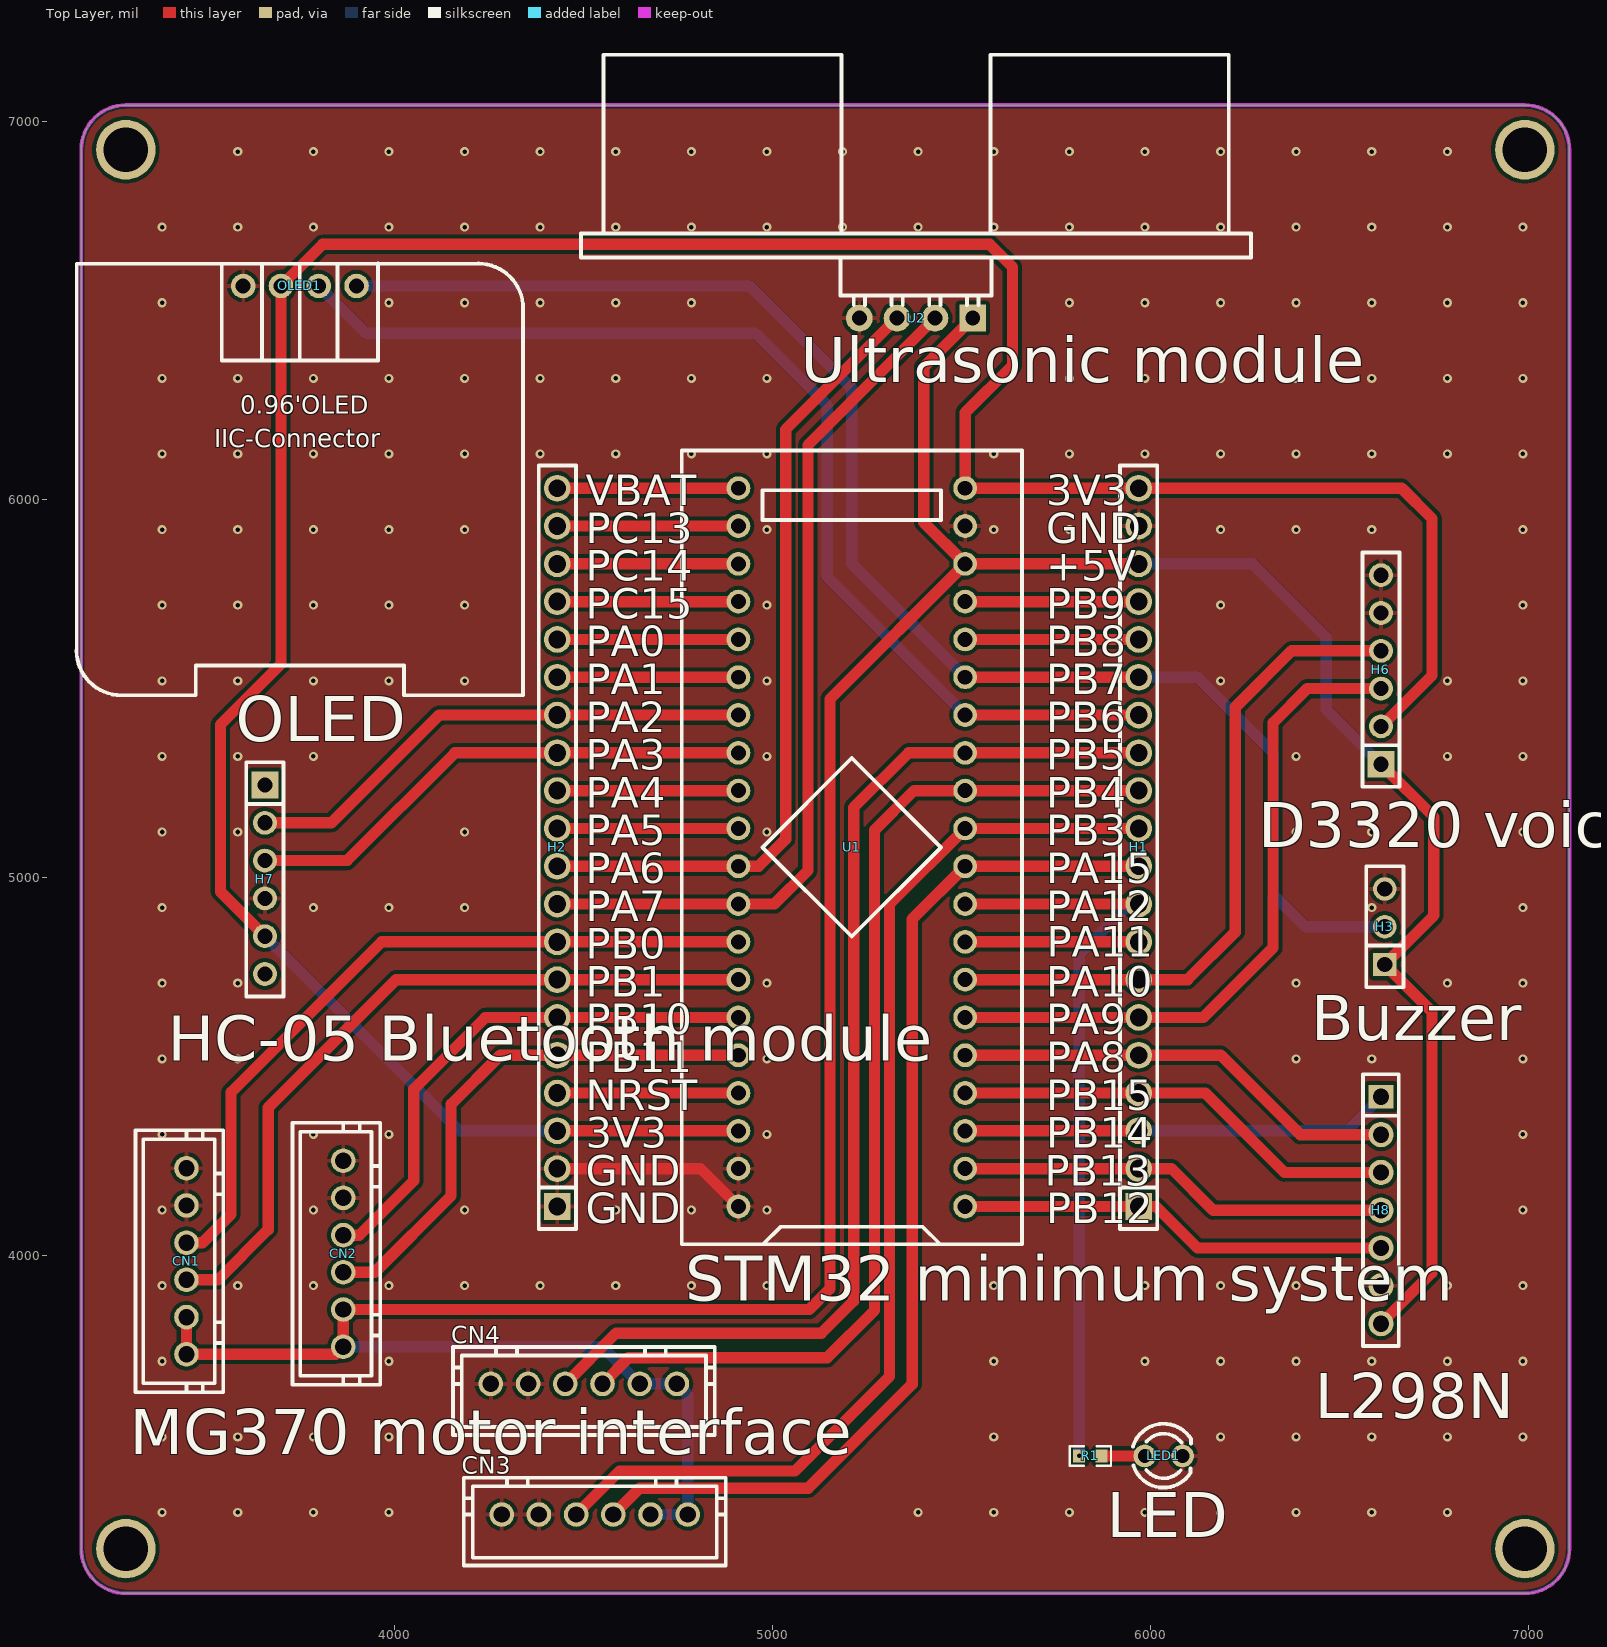
[diagram p0: Top Layer view]
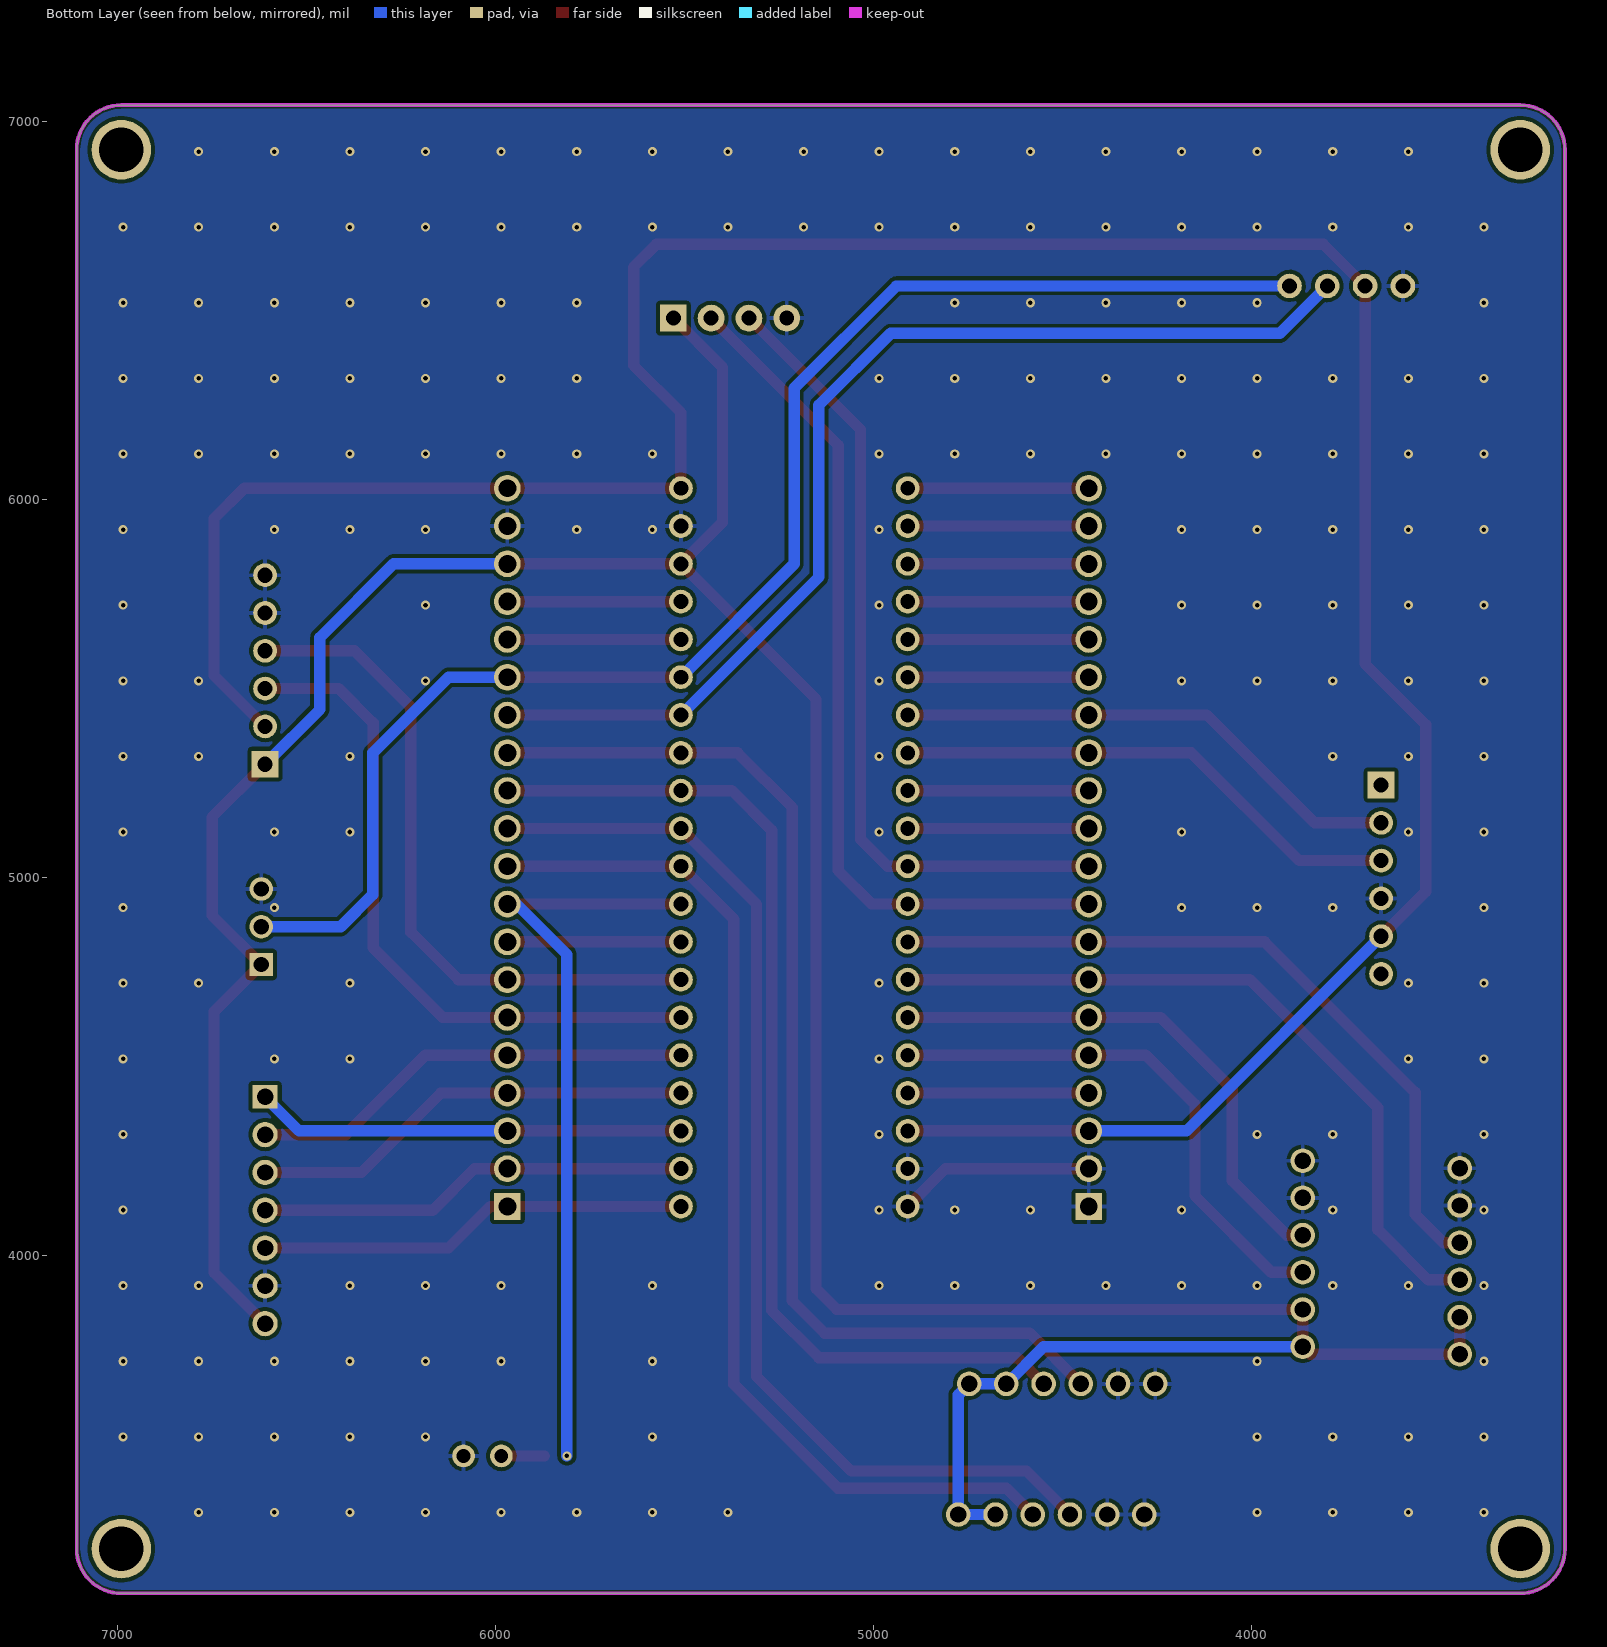
[diagram p1: Bottom Layer view, seen from below]
# Altium PCB MISC89099.pcbdoc
Units mil, origin at the board's own origin, x right, y up, seen from the top; angles counter-clockwise.
Board outline 3937.01 x 3937.01 mil, 2 copper layers (Top Layer, Bottom Layer), stack 62.206 mil thick; 15 components, 38 nets, 142 pads, 202 vias.

## Layer stack, top to bottom
Top Solder Mask Layer: solder mask 0.394, Dk 3.3
Top Layer: signal copper 1.379
Dielectric1: surface 59.449, FR4, Dk 4.5
Bottom Layer: signal copper 1.378
Bottom Solder Mask Layer: solder mask 0.394, Dk 3.3

## Board outline
3289.61,7043.5 ccw(c3289.61,6925.39) 3171.5,6925.39 3171.5,3224.61 ccw(c3289.61,3224.61) 3289.61,3106.5 6990.39,3106.5 ccw(c6990.39,3224.61) 7108.5,3224.61 7108.5,6925.39 ccw(c6990.39,6925.39) 6990.39,7043.5 3289.61,7043.5

## Design rules (kind name [scope] priority, off if disabled: settings)
BoardOutlineClearance copperThickness2oz_1 [All] p2 off: genericclearance=7.99 ignorepadtopadclearanceinfootprint=FALSE except(0: Arc-SplitContinuation Track-SplitContinuation SMDPad-SplitContinuation THPad-SplitContinuation Via-SplitContinuation Fill-SplitContinuation Region-SplitContinuation Poly-SplitContinuation Text-SplitContinuation Hole-SplitContinuation; 5.98: Arc-CutoutEdge Track-CutoutEdge SMDPad-CutoutEdge THPad-CutoutEdge Via-CutoutEdge Text-CutoutEdge; 6.9: Hole-OutlineEdge Hole-CutoutEdge; 10: Poly-OutlineEdge Poly-CutoutEdge; 11.81: Arc-OutlineEdge Track-OutlineEdge SMDPad-OutlineEdge THPad-OutlineEdge Via-OutlineEdge Fill-OutlineEdge Region-OutlineEdge Text-OutlineEdge Fill-CutoutEdge Region-CutoutEdge)
BoardOutlineClearance Plane_innerPlane_1 [All] p4 off: genericclearance=4.02 ignorepadtopadclearanceinfootprint=FALSE except(0: Arc-SplitContinuation Track-SplitContinuation SMDPad-SplitContinuation THPad-SplitContinuation Via-SplitContinuation Fill-SplitContinuation Region-SplitContinuation Poly-SplitContinuation Text-SplitContinuation Hole-SplitContinuation; 5.98: Arc-CutoutEdge Track-CutoutEdge SMDPad-CutoutEdge THPad-CutoutEdge Via-CutoutEdge Text-CutoutEdge; 6.9: Hole-OutlineEdge Hole-CutoutEdge; 10: Poly-OutlineEdge Poly-CutoutEdge; 11.81: Arc-OutlineEdge Track-OutlineEdge SMDPad-OutlineEdge THPad-OutlineEdge Via-OutlineEdge Fill-OutlineEdge Region-OutlineEdge Text-OutlineEdge Fill-CutoutEdge Region-CutoutEdge)
BoardOutlineClearance Copper_copperRegion_1 [All] p6 off: genericclearance=4.02 ignorepadtopadclearanceinfootprint=FALSE except(0: Arc-SplitContinuation Track-SplitContinuation SMDPad-SplitContinuation THPad-SplitContinuation Via-SplitContinuation Fill-SplitContinuation Region-SplitContinuation Poly-SplitContinuation Text-SplitContinuation Hole-SplitContinuation; 5.98: Arc-CutoutEdge Track-CutoutEdge SMDPad-CutoutEdge THPad-CutoutEdge Via-CutoutEdge Text-CutoutEdge; 6.9: Hole-OutlineEdge Hole-CutoutEdge; 10: Poly-OutlineEdge Poly-CutoutEdge; 11.81: Arc-OutlineEdge Track-OutlineEdge SMDPad-OutlineEdge THPad-OutlineEdge Via-OutlineEdge Fill-OutlineEdge Region-OutlineEdge Text-OutlineEdge Fill-CutoutEdge Region-CutoutEdge)
BoardOutlineClearance copperThickness1oz_1 [All] p8: genericclearance=4.02 ignorepadtopadclearanceinfootprint=FALSE except(0: Arc-SplitContinuation Track-SplitContinuation SMDPad-SplitContinuation THPad-SplitContinuation Via-SplitContinuation Fill-SplitContinuation Region-SplitContinuation Poly-SplitContinuation Text-SplitContinuation Hole-SplitContinuation; 5.98: Arc-CutoutEdge Track-CutoutEdge SMDPad-CutoutEdge THPad-CutoutEdge Via-CutoutEdge Text-CutoutEdge; 6.9: Hole-OutlineEdge Hole-CutoutEdge; 10: Poly-OutlineEdge Poly-CutoutEdge; 11.81: Arc-OutlineEdge Track-OutlineEdge SMDPad-OutlineEdge THPad-OutlineEdge Via-OutlineEdge Fill-OutlineEdge Region-OutlineEdge Text-OutlineEdge Fill-CutoutEdge Region-CutoutEdge)
Clearance copperThickness2oz [All] p1 off: gap=7.99 ignorepadtopadclearanceinfootprint=FALSE except(5.98: SMDPad-Track SMDPad-SMDPad THPad-Track SMDPad-THPad THPad-THPad Track-Via SMDPad-Via THPad-Via Via-Via Fill-SMDPad Region-SMDPad Fill-THPad Region-THPad Fill-Via Region-Via Fill-Fill Fill-Region Region-Region Arc-Track Arc-SMDPad Arc-THPad Arc-Via Fill-Arc Region-Arc Arc-Arc Text-Track SMDPad-Text Text-THPad Text-Via Fill-Text Region-Text Arc-Text Text-Text; 6.9: Hole-Track Hole-SMDPad Hole-THPad Hole-Via Fill-Hole Region-Hole Hole-Arc Hole-Text; 10: Poly-Track Poly-SMDPad Poly-THPad Poly-Via Poly-Fill Poly-Region Poly-Poly Poly-Arc Poly-Text Poly-Hole; 11.81: Fill-Track Region-Track)
Clearance Plane_innerPlane [All] p3 off: gap=4.02 ignorepadtopadclearanceinfootprint=FALSE except(5.98: SMDPad-Track SMDPad-SMDPad THPad-Track SMDPad-THPad THPad-THPad Track-Via SMDPad-Via THPad-Via Via-Via Fill-SMDPad Region-SMDPad Fill-THPad Region-THPad Fill-Via Region-Via Fill-Fill Fill-Region Region-Region Arc-Track Arc-SMDPad Arc-THPad Arc-Via Fill-Arc Region-Arc Arc-Arc Text-Track SMDPad-Text Text-THPad Text-Via Fill-Text Region-Text Arc-Text Text-Text; 6.9: Hole-Track Hole-SMDPad Hole-THPad Hole-Via Fill-Hole Region-Hole Hole-Arc Hole-Text; 10: Poly-Track Poly-SMDPad Poly-THPad Poly-Via Poly-Fill Poly-Region Poly-Poly Poly-Arc Poly-Text Poly-Hole; 11.81: Fill-Track Region-Track)
Clearance Copper_copperRegion [All] p5 off: gap=4.02 ignorepadtopadclearanceinfootprint=FALSE except(5.98: SMDPad-Track SMDPad-SMDPad THPad-Track SMDPad-THPad THPad-THPad Track-Via SMDPad-Via THPad-Via Via-Via Fill-SMDPad Region-SMDPad Fill-THPad Region-THPad Fill-Via Region-Via Fill-Fill Fill-Region Region-Region Arc-Track Arc-SMDPad Arc-THPad Arc-Via Fill-Arc Region-Arc Arc-Arc Text-Track SMDPad-Text Text-THPad Text-Via Fill-Text Region-Text Arc-Text Text-Text; 6.9: Hole-Track Hole-SMDPad Hole-THPad Hole-Via Fill-Hole Region-Hole Hole-Arc Hole-Text; 10: Poly-Track Poly-SMDPad Poly-THPad Poly-Via Poly-Fill Poly-Region Poly-Poly Poly-Arc Poly-Text Poly-Hole; 11.81: Fill-Track Region-Track)
Clearance copperThickness1oz [All] p7: gap=4.02 ignorepadtopadclearanceinfootprint=FALSE except(5.98: SMDPad-Track SMDPad-SMDPad THPad-Track SMDPad-THPad THPad-THPad Track-Via SMDPad-Via THPad-Via Via-Via Fill-SMDPad Region-SMDPad Fill-THPad Region-THPad Fill-Via Region-Via Fill-Fill Fill-Region Region-Region Arc-Track Arc-SMDPad Arc-THPad Arc-Via Fill-Arc Region-Arc Arc-Arc Text-Track SMDPad-Text Text-THPad Text-Via Fill-Text Region-Text Arc-Text Text-Text; 6.9: Hole-Track Hole-SMDPad Hole-THPad Hole-Via Fill-Hole Region-Hole Hole-Arc Hole-Text; 10: Poly-Track Poly-SMDPad Poly-THPad Poly-Via Poly-Fill Poly-Region Poly-Poly Poly-Arc Poly-Text Poly-Hole; 11.81: Fill-Track Region-Track)
DiffPairsRouting differentialPair [All] p1: maxlimit=6 minlimit=6 mostfreqgap=6 toplayer_minwidth=5 toplayer_prefwidth=10 toplayer_maxwidth=100 toplayer_mingap=6 toplayer_prefgap=6 toplayer_maxgap=6 bottomlayer_minwidth=5 bottomlayer_prefwidth=10 bottomlayer_maxwidth=100 bottomlayer_mingap=6 bottomlayer_prefgap=6 bottomlayer_maxgap=6 maxuncoupledlength=10
HoleToHoleClearance otherClearance [All] p1: gap=11.81 allowstackedmicrovias=TRUE
Length netLength [All] p1: minlimit=0 maxlimit=0
PasteMaskExpansion pasteMaskExpansion [All] p1: expansion=0
PlaneConnect innerPlane [All] p1: planeconnectstyle=Relief reliefexpansion=20 reliefentries=4 reliefconductorwidth=10 reliefairgap=10
PolygonConnect copperRegion [All] p1: connectstyle=Relief reliefconductorwidth=10 reliefentries=4 polygonreliefangle="90 Angle" airgapwidth=10 via.connectstyle=Relief via.reliefconductorwidth=10 via.reliefentries=4 via.polygonreliefangle="90 Angle" via.airgapwidth=10
RoutingVias viaSize [All] p1: holewidth=12.01 width=24.02 viastyle="Through Hole" minholewidth=11.81 minwidth=19.68 maxholewidth=248.03 maxwidth=393.7
SolderMaskExpansion solderMaskExpansion [IsVia] p1: expansion=-1000 istentingtop=TRUE
SolderMaskExpansion solderMaskExpansion [All] p2: expansion=2 istentingtop=FALSE
Width copperThickness2oz_2 [All] p1 off: maxlimit=100 minlimit=8 preferedwidth=10
Width copperThickness1oz_2 [All] p2: maxlimit=100 minlimit=5 preferedwidth=10

## Components (designator, comment, footprint, x,y, rotation, side; value= is the part's Value field where it differs from the comment)
CN1 "XH2.54*6P_through-hole" CONN-TH_XH2.54-6P 3450,3985 r270 top
CN2 "XH2.54*6P_through-hole" CONN-TH_XH2.54-6P 3865,4005 r270 top
CN3 "XH2.54*6P_through-hole" CONN-TH_XH2.54-6P 4530,3315 r0 top
CN4 "XH2.54*6P_through-hole" CONN-TH_XH2.54-6P 4501.36,3660.61 r0 top
H1 "" HDR-TH_20P-P2.54-V-F 5969.16,5080 r90 top
H2 "" HDR-TH_20P-P2.54-V-F 4430.95,5080 r90 top
H3 "" HDR-TH_3P-P2.54-V-F 6620,4870 r90 top
H6 "" HDR-TH_6P-P2.54-V-F 6610,5550 r90 top
H7 "" HDR-TH_6P-P2.54-V-F 3657.66,4995 r270 top
H8 "" HDR-TH_7P-P2.54-V-F 6610.01,4120 r270 top
LED1 "" LED_TH-3mm 6035,3470 r0 top
OLED1 "" 0.96OLED_4P 3750,6565 r0 top
R1 "220" R0603 5841.36,3469.92 r180 top
U1 "STM32F103C8T6-Card" CONN-TH_L53.3-W22.9_STM32F103C8T6-CARD 5210,5080 r90 top
U2 "HC-SR04" TH_HC-SR04V 5380,6480 r180 top

## Footprints (in the part's own frame and the unit in brackets; to place one, negate y for a bottom-side part, rotate by r counter-clockwise, add the part's x,y. Pads: shape width x height; smd on the part's side, far side on the other; paste and mask are expansions set on the pad)
0.96OLED_4P [mm]
  round 1.65 hole 1 copper offset 0,0: 1(-3.81,-0.001) 2(-1.27,0.002) 3(1.27,0.002) 4(3.81,0.002)
  silkscreen extent -15,-27.5 15,1.5
CONN-TH_L53.3-W22.9_STM32F103C8T6-CARD [mm]
  round 1.6 hole 1: 1(-24.13,-7.62) 2(-21.59,-7.62) 3(-19.05,-7.62) 4(-16.51,-7.62) 5(-13.97,-7.62) 6(-11.43,-7.62) 7(-8.89,-7.62) 8(-6.35,-7.62) 9(-3.81,-7.62) 10(-1.27,-7.62) 11(1.27,-7.62) 12(3.81,-7.62) 13(6.35,-7.62) 14(8.89,-7.62) 15(11.43,-7.62) 16(13.97,-7.62) 17(16.51,-7.62) 18(19.05,-7.62) 19(21.59,-7.62) 20(24.13,-7.62) 21(24.13,7.62) 22(21.59,7.62) 23(19.05,7.62) 24(16.51,7.62) 25(13.97,7.62) 26(11.43,7.62) 27(8.89,7.62) 28(6.35,7.62) 29(3.81,7.62) 30(1.27,7.62) 31(-1.27,7.62) 32(-3.81,7.62) 33(-6.35,7.62) 34(-8.89,7.62) 35(-11.43,7.62) 36(-13.97,7.62) 37(-16.51,7.62) 38(-19.05,7.62) 39(-21.59,7.62) 40(-24.13,7.62)
  silkscreen extent -26.67,-11.43 26.67,11.43
CONN-TH_XH2.54-6P [mm]
  round 1.65 hole 1.1 paste+0 mask+0.05: 1(-6.25,0) 2(-3.75,0) 3(-1.25,0) 4(1.25,0) 5(3.75,0) 6(6.25,0)
  silkscreen extent -8.8,-3.43 8.8,2.47
HDR-TH_3P-P2.54-V-F [mil]
  rect 62x62 hole 40.16: 1(-100,0)
  round 62 hole 40.16: 2(0,0) 3(100,0)
  silkscreen extent -160,-49 160,49
HDR-TH_6P-P2.54-V-F [mm]
  rect 1.8x1.8 hole 1.02: 1(-6.35,0)
  round 1.6 hole 1.02: 2(-3.81,0) 3(-1.27,0) 4(1.27,0) 5(3.81,0) 6(6.35,0)
  silkscreen extent -7.87,-1.25 7.87,1.25
HDR-TH_7P-P2.54-V-F [mm]
  rect 1.575x1.7 hole 1.1: 1(-7.62,0)
  round 1.7 hole 1.1: 2(-5.08,0) 3(-2.54,0) 4(0,0) 5(2.54,0) 6(5.08,0) 7(7.62,0)
  silkscreen extent -9.13,-1.2 9.13,1.2
HDR-TH_20P-P2.54-V-F [mm]
  rect 1.8x1.8 hole 1.2: 1(-24.13,0)
  round 1.8 hole 1.2: 2(-21.59,0) 3(-19.05,0) 4(-16.51,0) 5(-13.97,0) 6(-11.43,0) 7(-8.89,0) 8(-6.35,0) 9(-3.81,0) 10(-1.27,0) 11(1.27,0) 12(3.81,0) 13(6.35,0) 14(8.89,0) 15(11.43,0) 16(13.97,0) 17(16.51,0) 18(19.05,0) 19(21.59,0) 20(24.13,0)
  silkscreen extent -25.65,-1.25 25.65,1.25
LED_TH-3mm [mil]
  round 60 hole 36 paste+0 mask+2: 1(-50,0) 2(50,0)
  silkscreen extent -81,-84 72,85
R0603 [mil]
  rect 31.75x34.02 smd paste-3937.01 mask+2: 1(-29.66,0) 2(29.66,0)
  silkscreen extent -55,-26 55,26
TH_HC-SR04V [mm]
  rect 1.8x1.8 hole 1.001: 1(-3.81,0)
  round 1.8 hole 1.001: 2(-1.27,0) 3(1.27,0) 4(3.81,0)
  silkscreen extent -22.5,-17.7 22.5,-0.89

## Free pads (board coordinates)
  round 157.48 hole 118.11: 1(3289.61,6925.39) 1(3289.61,3224.61) 1(6990.39,6925.39) 1(6990.39,3224.61)

## Via types
v1: diameter 24.02, hole 12, Top Layer to Bottom Layer, 202 vias

## Nets (pads, with @x,y where several pads share a name; then routed paths per layer and width w, separated by ;. In a path a pad name is that pad's centre, name@x,y a point inside that pad or via, vN(x,y) a via of type N, cw(c..) or ccw(c..) an arc to the next point about the centre after c; other vN are vias at no path point)
$1N17006: LED1.1 R1.1 | length 114
  Top Layer w30: R1.1 5871.1,3470 LED1.1
+5V: CN1.5 CN1.6 CN2.5 CN2.6 CN3.5 CN3.6 CN4.5 CN4.6 H1.18 H3.1 H6.1 H8.7 U1.18 U2.1 | length 9254.9
  Top Layer w30: CN1.5 CN1.6 3845,3738.94 CN2.6 CN2.5 5097.36,3857.36 5152.6,3912.6 5152.6,5472.61 U1.18 ; U2.1 5400,6350 5400,5940 U1.18 ; H1.18 U1.18 ; H8.7 6745,3954.99 6745,4645 H3.1 6750,4900 6750,5160 H6.1
  Bottom Layer w30: CN2.6 4550.67,3758.94 CN4.5 CN4.6 4776.06,3631.97 CN3.6 CN3.5 ; H1.18 6270,5830 6465,5635 6465,5445 H6.1
ENA: H1.3 H8.1 U1.3 | length 1137.3
  Top Layer w30: U1.3 H1.3
  Bottom Layer w30: H1.3 6520.01,4330 H8.1
GND: CN1.1 CN1.2 CN2.1 CN2.2 CN3.1 CN3.2 CN4.1 CN4.2 H1.19 H2.1 H2.2 H3.3 H6.5 H6.6 H7.4 H8.6 LED1.2 OLED1.1 U1.19 U1.39 U1.40 U2.4 | length 520.5
  Top Layer w30: H2.2 4810,4230 U1.40
  other v1: 3385.6,3320.6 3585.6,3320.6 3785.6,3320.6 3985.6,3320.6 5385.6,3320.6 5585.6,3320.6 5785.6,3320.6 5985.6,3320.6 6185.6,3320.6 6385.6,3320.6 6585.6,3320.6 6785.6,3320.6 3385.6,3520.6 3585.6,3520.6 3785.6,3520.6 3985.6,3520.6 5585.6,3520.6 6185.6,3520.6 6385.6,3520.6 6585.6,3520.6 6785.6,3520.6 6985.6,3520.6 3385.6,3720.6 3985.6,3720.6 5585.6,3720.6 5985.6,3720.6 6185.6,3720.6 6385.6,3720.6 6585.6,3720.6 6785.6,3720.6 6985.6,3720.6 3385.6,3920.6 3585.6,3920.6 3785.6,3920.6 3985.6,3920.6 4185.6,3920.6 4385.6,3920.6 4585.6,3920.6 4785.6,3920.6 4985.6,3920.6 5585.6,3920.6 5985.6,3920.6 6185.6,3920.6 6385.6,3920.6 6785.6,3920.6 6985.6,3920.6 3385.6,4120.6 3785.6,4120.6 4185.6,4120.6 4585.6,4120.6 4785.6,4120.6 4985.6,4120.6 6985.6,4120.6 3385.6,4320.6 3785.6,4320.6 3985.6,4320.6 4985.6,4320.6 6985.6,4320.6 3385.6,4520.6 3585.6,4520.6 4985.6,4520.6 6385.6,4520.6 6585.6,4520.6 6985.6,4520.6 3385.6,4720.6 3585.6,4720.6 4985.6,4720.6 6385.6,4720.6 6785.6,4720.6 6985.6,4720.6 3385.6,4920.6 3785.6,4920.6 3985.6,4920.6 4185.6,4920.6 6585.6,4920.6 6985.6,4920.6 3385.6,5120.6 3585.6,5120.6 4185.6,5120.6 4985.6,5120.6 6385.6,5120.6 6585.6,5120.6 6985.6,5120.6 3385.6,5320.6 3585.6,5320.6 3785.6,5320.6 4985.6,5320.6 6385.6,5320.6 6785.6,5320.6 6985.6,5320.6 3385.6,5520.6 3585.6,5520.6 3785.6,5520.6 3985.6,5520.6 4185.6,5520.6 4985.6,5520.6 6185.6,5520.6 6785.6,5520.6 6985.6,5520.6 3385.6,5720.6 3585.6,5720.6 3785.6,5720.6 3985.6,5720.6 4185.6,5720.6 4985.6,5720.6 6185.6,5720.6 6985.6,5720.6 3385.6,5920.6 3585.6,5920.6 3785.6,5920.6 3985.6,5920.6 4185.6,5920.6 4985.6,5920.6 5585.6,5920.6 5785.6,5920.6 6185.6,5920.6 6385.6,5920.6 6585.6,5920.6 6985.6,5920.6 3385.6,6120.6 3585.6,6120.6 3785.6,6120.6 3985.6,6120.6 4185.6,6120.6 4385.6,6120.6 4585.6,6120.6 4785.6,6120.6 4985.6,6120.6 5585.6,6120.6 5785.6,6120.6 5985.6,6120.6 6185.6,6120.6 6385.6,6120.6 6585.6,6120.6 6785.6,6120.6 6985.6,6120.6 3385.6,6320.6 3585.6,6320.6 3785.6,6320.6 3985.6,6320.6 4185.6,6320.6 4385.6,6320.6 4585.6,6320.6 4785.6,6320.6 4985.6,6320.6 5785.6,6320.6 5985.6,6320.6 6185.6,6320.6 6385.6,6320.6 6585.6,6320.6 6785.6,6320.6 6985.6,6320.6 3385.6,6520.6 3985.6,6520.6 4185.6,6520.6 4385.6,6520.6 4585.6,6520.6 4785.6,6520.6 5785.6,6520.6 5985.6,6520.6 6185.6,6520.6 6385.6,6520.6 6585.6,6520.6 6785.6,6520.6 6985.6,6520.6 3385.6,6720.6 3585.6,6720.6 3785.6,6720.6 3985.6,6720.6 4185.6,6720.6 4385.6,6720.6 4585.6,6720.6 4785.6,6720.6 4985.6,6720.6 5185.6,6720.6 5385.6,6720.6 5585.6,6720.6 5785.6,6720.6 5985.6,6720.6 6185.6,6720.6 6385.6,6720.6 6585.6,6720.6 6785.6,6720.6 6985.6,6720.6 3585.6,6920.6 3785.6,6920.6 3985.6,6920.6 4185.6,6920.6 4385.6,6920.6 4585.6,6920.6 4785.6,6920.6 4985.6,6920.6 5185.6,6920.6 5385.6,6920.6 5585.6,6920.6 5785.6,6920.6 5985.6,6920.6 6185.6,6920.6 6385.6,6920.6 6585.6,6920.6 6785.6,6920.6
IN1: H1.5 H8.2 U1.5 | length 1187
  Top Layer w30: U1.5 H1.5 6186.42,4530 6396.42,4320 H8.2
IN2: H1.4 H8.3 U1.4 | length 1187
  Top Layer w30: U1.4 H1.4 6145,4430 6355,4220 H8.3
IN3: H1.2 H8.4 U1.2 | length 1145.6
  Top Layer w30: U1.2 H1.2 6056.01,4230 6166.01,4120 H8.4
IN4: H1.1 H8.5 U1.1 | length 1145.6
  Top Layer w30: U1.1 H1.1 6014.59,4130 6124.59,4020 H8.5
NRST: H2.4 U1.37 | length 479
  Top Layer w30: H2.4 U1.37
PA0: H2.16 U1.25 | length 479
  Top Layer w30: H2.16 U1.25
PA1: H2.15 U1.26 | length 479
  Top Layer w30: H2.15 U1.26
PA2: H2.14 H7.2 U1.27 | length 1370.4
  Top Layer w30: H7.2 3833.58,5145 4118.58,5430 H2.14 U1.27
PA3: H2.13 H7.3 U1.28 | length 1370.4
  Top Layer w30: H7.3 3875,5045 4160,5330 H2.13 U1.28
PA4: H2.12 U1.29 | length 479
  Top Layer w30: H2.12 U1.29
PA5: H2.11 U1.30 | length 479
  Top Layer w30: H2.11 U1.30
PA6: H2.10 U1.31 U2.3 | length 2134.4
  Top Layer w30: H2.10 U1.31 4963.58,5030 5035,5101.42 5035,6185 U2.3
PA7: H2.9 U1.32 U2.2 | length 2300.1
  Top Layer w30: H2.9 U1.32 5005,4930 5094.02,5019.02 5094.02,6144.02 U2.2
PA9: H1.6 H6.3 U1.6 | length 1808.9
  Top Layer w30: U1.6 H1.6 6140,4630 6324.29,4814.29 6324.29,5409.29 6415,5500 H6.3
PA10: H1.7 H6.4 U1.7 | length 1808.9
  Top Layer w30: U1.7 H1.7 6098.58,4730 6224.29,4855.71 6224.29,5450.71 6373.58,5600 H6.4
PA11: H1.8 U1.8 | length 459.2
  Top Layer w30: U1.8 H1.8
PA12: H1.9 R1.2 U1.9 | length 1998.6
  Top Layer w30: U1.9 H1.9
  Bottom Layer w30: v1(5811.7,3469.92) 5811.7,4796.7 5945,4930 H1.9
PA15: CN3.4 H1.10 U1.10 | length 2820.8
  Top Layer w30: CN3.4 4649.21,3385 5095,3385 5370,3660 5370,4890 U1.10 H1.10
PB0: CN1.3 H2.8 U1.33 | length 1978.5
  Top Layer w30: CN1.3 3492.48,4034.21 3567.71,4109.44 3567.71,4431.89 3965.82,4830 H2.8 U1.33
PB1: CN1.4 H2.7 U1.34 | length 1977.9
  Top Layer w30: CN1.4 3533.25,3935.79 3666.13,4068.67 3666.13,4391.13 4005,4730 H2.7 U1.34
PB3: CN3.3 H1.11 U1.11 | length 2972.4
  Top Layer w30: CN3.3 4595.79,3430 5060,3430 5310,3680 5310,4930 U1.11 H1.11
PB4: CN4.4 H1.12 U1.12 | length 2812.6
  Top Layer w30: CN4.4 4619.96,3730 5145,3730 5270,3855 5270,5125 5375,5230 U1.12 H1.12
PB5: CN4.3 H1.13 U1.13 | length 2972.9
  Top Layer w30: CN4.3 4586.54,3795 5130,3795 5215,3880 5215,5185 5360,5330 U1.13 H1.13
PB6: H1.14 OLED1.3 U1.14 | length 2905.8
  Top Layer w30: U1.14 H1.14
  Bottom Layer w30: OLED1.3@3800,6565.05 3925.05,6440 4955,6440 5145,6250 5145,5795 U1.14
PB7: H1.15 H3.2 OLED1.4 U1.15 | length 3914.2
  Top Layer w30: U1.15 H1.15
  Bottom Layer w30: OLED1.4@3900,6565.05 4939.95,6565.05 5210,6295 5210,5830 U1.15 ; H1.15 6125,5530 6325,5330 6325,4955 6410,4870 H3.2
PB8: H1.16 U1.16 | length 459.2
  Top Layer w30: U1.16 H1.16
PB9: H1.17 U1.17 | length 459.2
  Top Layer w30: U1.17 H1.17
PB10: CN2.3 H2.6 U1.35 | length 1425.5
  Top Layer w30: CN2.3 3907.48,4054.21 4051.58,4198.31 4051.58,4440.77 4240.82,4630 H2.6 U1.35
PB11: CN2.4 H2.5 U1.36 | length 1424.9
  Top Layer w30: CN2.4 3948.25,3955.79 4150,4157.54 4150,4400 4280,4530 H2.5 U1.36
PC13: H2.19 U1.22 | length 479
  Top Layer w30: H2.19 U1.22
PC14: H2.18 U1.23 | length 479
  Top Layer w30: H2.18 U1.23
PC15: H2.17 U1.24 | length 479
  Top Layer w30: H2.17 U1.24
VBAT: H2.20 U1.21 | length 479
  Top Layer w30: H2.20 U1.21
VCC: H1.20 H2.3 H6.2 H7.5 OLED1.2 U1.20 U1.38 | length 7816.9
  Top Layer w30: H7.5 3540,4962.66 3540,5405 3700,5565 3700,6565.05 3809.95,6675 5575,6675 5635,6615 5635,6355 5510,6230 U1.20 H1.20 6665,6030 6745,5950 6745,5535 H6.2 ; H2.3 U1.38
  Bottom Layer w30: H7.5 4172.66,4330 H2.3
pads on no net: H7.1 H7.6

## Polygon pours and split planes (outlines as drawn)
GND on Bottom Layer (solid, remove dead copper, pour order 2): 3100,7165 3100,3000 7275,3000 7275,7165
GND on Top Layer (solid, remove dead copper, pour order 0): 3000,7145 3000,3075 7385,3075 7385,7145

## Keep-outs
Board Outline Layer:
  the board outline again, w10

## Silkscreen, mask and mechanical layers (free items; w line width, h text height)
Top Silkscreen Layer:
  text "Ultrasonic module" at 5075,6310 h120
  text "VBAT" at 4505.95,5985 h80
  text "3V3" at 5724.16,5985 h80
  text "PC13" at 4505.95,5885 h80
  text "GND" at 5724.16,5885 h80
  text "PC14" at 4505.95,5785 h80
  text "+5V" at 5724.16,5785 h80
  text "PC15" at 4505.95,5685 h80
  text "PB9" at 5724.16,5685 h80
  text "PA0" at 4505.95,5585 h80
  text "PB8" at 5724.16,5585 h80
  text "PA1" at 4505.95,5485 h80
  text "PB7" at 5724.16,5485 h80
  text "PA2" at 4505.95,5385 h80
  text "PB6" at 5724.16,5385 h80
  text "OLED" at 3580,5360 h120
  text "PA3" at 4505.95,5285 h80
  text "PB5" at 5724.16,5285 h80
  text "PA4" at 4505.95,5185 h80
  text "PB4" at 5724.16,5185 h80
  text "PA5" at 4505.95,5085 h80
  text "PB3" at 5724.16,5085 h80
  text "D3320 voice recognition" at 6285,5080 h120
  text "PA6" at 4505.95,4985 h80
  text "PA15" at 5724.16,4985 h80
  text "PA7" at 4505.95,4885 h80
  text "PA12" at 5724.16,4885 h80
  text "PA11" at 5725.95,4790 h80
  text "PB0" at 4505.95,4785 h80
  text "PB1" at 4505.95,4685 h80
  text "PA10" at 5724.16,4685 h80
  text "PB10" at 4505.95,4585 h80
  text "PA9" at 5724.16,4585 h80
  text "Buzzer" at 6425,4570 h120
  text "HC-05 Bluetooth module" at 3400,4515 h120
  text "PB11" at 4505.95,4485 h80
  text "PA8" at 5724.16,4485 h80
  text "NRST" at 4505.95,4385 h80
  text "PB15" at 5724.16,4385 h80
  text "3V3" at 4505.95,4285 h80
  text "PB14" at 5724.16,4285 h80
  text "GND" at 4505.95,4185 h80
  text "PB13" at 5720.95,4185 h80
  text "GND" at 4505.95,4085 h80
  text "PB12" at 5724.16,4085 h80
  text "STM32 minimum system" at 4770,3880 h120
  text "L298N" at 6435,3570 h120
  text "MG370 motor interface" at 3300,3475 h120
  text "LED" at 5885,3255 h120